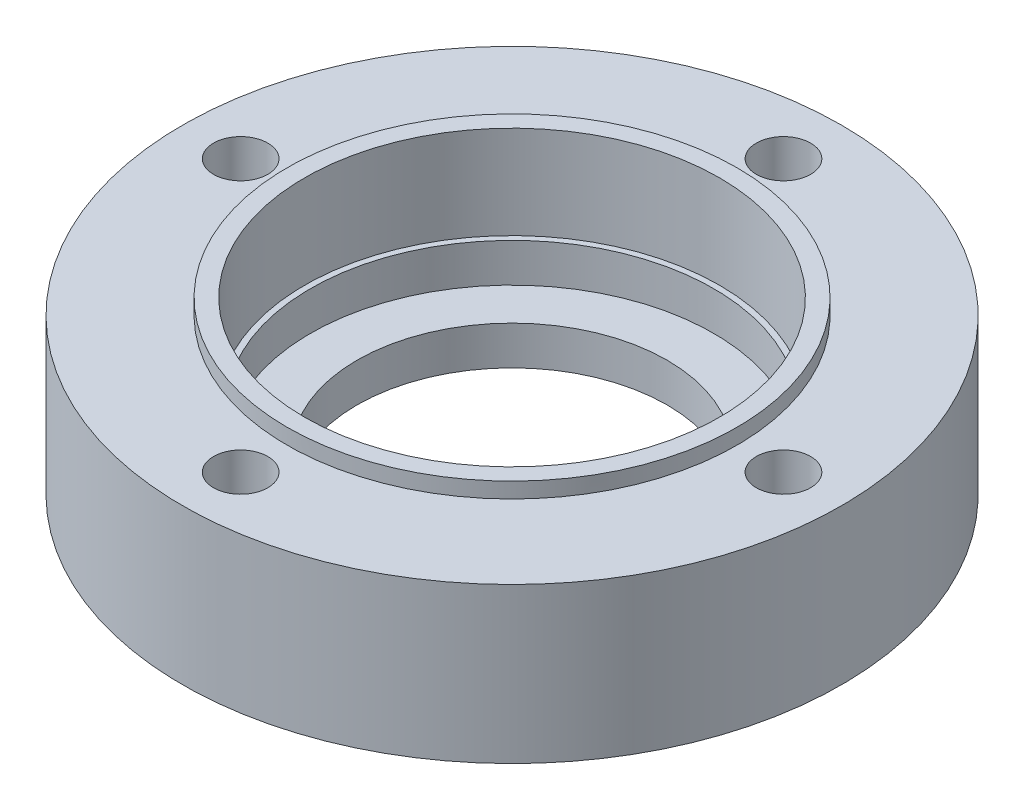
from build123d import *

# Parameters (mm, degrees)
SKETCH1_R            = 42.5
SKETCH1_R_2          = 20
BOSS_EXTRUDE1_DEPTH  = 20
M6_CLEARANCE_HOLE1_D = 7
SKETCH4_R            = 26
CUT_EXTRUDE1_DEPTH   = 15
SKETCH5_R            = 29
SKETCH5_R_2          = 26.75
BOSS_EXTRUDE3_DEPTH  = 2
CUT_EXTRUDE2_START   = -12
SKETCH6_R            = 26.75
CUT_EXTRUDE2_DEPTH   = 12
SKETCH7_R            = 5.5
CUT_EXTRUDE3_DEPTH   = 7


with BuildPart() as part:
    # Sketch1 → Boss-Extrude1 (new body)
    with BuildSketch(Plane.XZ):
        with Locations(Location((0, 0, 0), (0, 0, 270))):
            Circle(SKETCH1_R)
        with Locations(Location((0, 0, 0), (0, 0, 270))):
            Circle(SKETCH1_R_2, mode=Mode.SUBTRACT)
    extrude(amount=BOSS_EXTRUDE1_DEPTH)

    # M6 Clearance Hole1 (through all)
    with Locations(Plane(origin=(0, 0, 0), x_dir=(1, 0, 0), z_dir=(0, 1, 0))):
        with Locations((0, -35), (0, 35), (-35, 0), (35, 0)):
            Hole(M6_CLEARANCE_HOLE1_D / 2)

    # Sketch4 → Cut-Extrude1 (cut)
    with BuildSketch(Plane(origin=(0, 0, 0), x_dir=(1, 0, 0), z_dir=(0, 1, 0))):
        with Locations(Location((0, 0, 0), (0, 0, 270))):
            Circle(SKETCH4_R)
    extrude(amount=-CUT_EXTRUDE1_DEPTH, mode=Mode.SUBTRACT)

    # Sketch5 → Boss-Extrude3 (add)
    with BuildSketch(Plane(origin=(0, 0, 0), x_dir=(1, 0, 0), z_dir=(0, 1, 0))):
        with Locations(Location((0, 0, 0), (0, 0, 90))):
            Circle(SKETCH5_R)
        with Locations(Location((0, 0, 0), (0, 0, 270))):
            Circle(SKETCH5_R_2, mode=Mode.SUBTRACT)
    extrude(amount=BOSS_EXTRUDE3_DEPTH)

    # Sketch6 → Cut-Extrude2 (cut)
    with BuildSketch(Plane(origin=(0, 2, 0), x_dir=(1, 0, 0), z_dir=(0, 1, 0)).offset(CUT_EXTRUDE2_START)):
        with Locations(Location((0, 0, 0), (0, 0, 270))):
            Circle(SKETCH6_R)
    extrude(amount=CUT_EXTRUDE2_DEPTH, mode=Mode.SUBTRACT)

    # Sketch7 → Cut-Extrude3 (cut)
    with BuildSketch(Plane.XZ.offset(20)):
        with Locations(Location((0, 35, 0), (0, 0, 270))):
            Circle(SKETCH7_R)
        with Locations(Location((-35, 0, 0), (0, 0, 270))):
            Circle(SKETCH7_R)
        with Locations(Location((0, -35, 0), (0, 0, 270))):
            Circle(SKETCH7_R)
        with Locations(Location((35, 0, 0), (0, 0, 270))):
            Circle(SKETCH7_R)
    extrude(amount=-CUT_EXTRUDE3_DEPTH, mode=Mode.SUBTRACT)


solid = part.part
